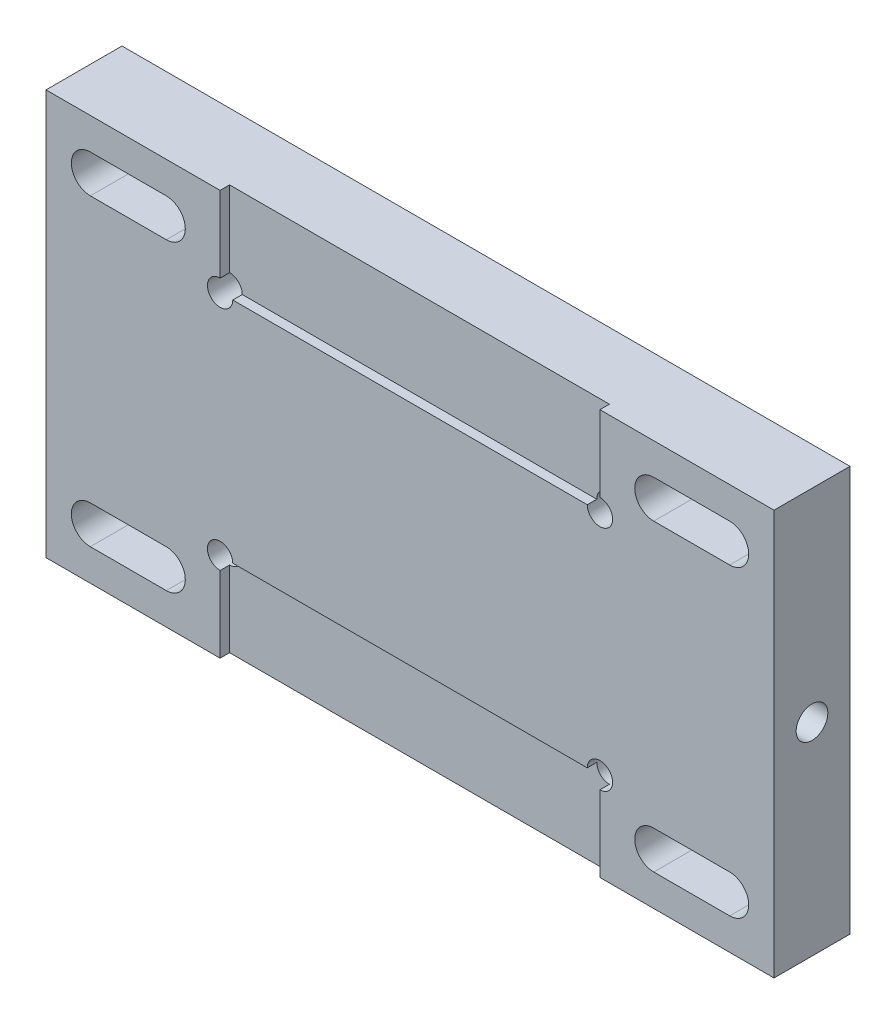
SolidWorks part; units mm, degrees
ref_plane "前视基准面" through (0, 0, 0) normal (0, 0, 1) x (1, 0, 0)
ref_plane "上视基准面" through (0, 0, 0) normal (0, 1, 0) x (1, 0, 0)
ref_plane "右视基准面" through (0, 0, 0) normal (1, 0, 0) x (0, 0, -1)
sketch "草图1" plane through (0, 0, 0) normal (0, 0, 1) x (1, 0, 0)
  line L1 (-57.5, -32) -> (57.5, -32)
  line L2 (-57.5, -32) -> (-57.5, 32)
  line L3 (-57.5, 32) -> (57.5, 32)
  line L4 (57.5, -32) -> (57.5, 32)
  line L5 (-57.5, -32) -> (57.5, 32) construction
  line L6 (-57.5, 32) -> (57.5, -32) construction
  point P0 (0, 0)
  dimension "D1" = 64
  dimension "D2" = 115
extrude "凸台-拉伸1" add sketch "草图1" along normal mid plane 12
sketch "草图2" plane through (0, 0, 6) normal (0, 0, 1) x (1, 0, 0)
  line L0 (57.5, 32) -> (-57.5, 32) construction
  line L1 (-30, 18) -> (30, 18)
  line L2 (-30, 18) -> (-30, 32)
  line L3 (-30, 32) -> (30, 32)
  line L4 (30, 18) -> (30, 32)
  line L5 (-30, 18) -> (30, 32) construction
  line L6 (-30, 32) -> (30, 18) construction
  point P0 (0, 25)
  dimension "D1" = 60
  dimension "D2" = 14
extrude "切除-拉伸1" cut sketch "草图2" against normal blind 1.5
sketch "草图3" plane through (0, 0, 6) normal (0, 0, 1) x (1, 0, 0)
  circle A0 centre (-30, 18) radius 2
  circle A1 centre (30, 18) radius 2
  dimension "D1" = 4
extrude "切除-拉伸2" cut sketch "草图3" against normal through all both and the other way through all
mirror "镜向1" about plane through (0, 0, 0) normal (0, 1, 0) of "切除-拉伸2", "切除-拉伸1"
sketch "草图4" plane through (0, 0, 6) normal (0, 0, 1) x (1, 0, 0)
  line L0 (-50.5, 24) -> (-38.5, 24) construction
  line L1 (-50.5, 27) -> (-38.5, 27)
  line L2 (-50.5, 21) -> (-38.5, 21)
  line L3 (-30, 32) -> (-57.5, 32) construction
  line L4 (-57.5, 32) -> (-57.5, -32) construction
  line L5 (0, 0) -> (0, 32) construction
  line L6 (30, 32) -> (-30, 32) construction
  line L7 (0, 0) -> (-57.5, 0) construction
  line L8 (50.5, 24) -> (38.5, 24) construction
  line L9 (50.5, 27) -> (38.5, 27)
  line L10 (50.5, 21) -> (38.5, 21)
  line L11 (-50.5, -24) -> (-38.5, -24) construction
  line L12 (-50.5, -27) -> (-38.5, -27)
  line L13 (-50.5, -21) -> (-38.5, -21)
  line L14 (50.5, -24) -> (38.5, -24) construction
  line L15 (50.5, -27) -> (38.5, -27)
  line L16 (50.5, -21) -> (38.5, -21)
  arc A0 (-50.5, 27) -> (-50.5, 21) centre (-50.5, 24) ccw
  arc A1 (-38.5, 21) -> (-38.5, 27) centre (-38.5, 24) ccw
  arc A2 (50.5, 27) -> (50.5, 21) centre (50.5, 24) cw
  arc A3 (38.5, 21) -> (38.5, 27) centre (38.5, 24) cw
  arc A4 (-50.5, -27) -> (-50.5, -21) centre (-50.5, -24) cw
  arc A5 (-38.5, -21) -> (-38.5, -27) centre (-38.5, -24) cw
  arc A6 (50.5, -27) -> (50.5, -21) centre (50.5, -24) ccw
  arc A7 (38.5, -21) -> (38.5, -27) centre (38.5, -24) ccw
  point P2 (-44.5, 24)
  point P19 (44.5, 24)
  point P26 (-44.5, -24)
  point P33 (44.5, -24)
  dimension "D1" = 3
  dimension "D2" = 12
  dimension "D3" = 5
  dimension "D4" = 7
extrude "切除-拉伸3" cut sketch "草图4" against normal up to next
hole_wizard "M6 螺纹孔1" positions "3D草图1" profile "草图5" tap size "M6" standard "GB"
sketch3d "3D草图1"
  line L0 (57.5, 0, 6) -> (57.5, 0, -6)
  line L1 (57.5, -32, 6) -> (57.5, 32, 6) construction
  line L2 (57.5, -32, -6) -> (57.5, 32, -6) construction
  point P0 (57.5, 0, 0)
sketch "草图5" plane through (57.5, 0, 0) normal (0, 1, 0) x (0, 0, -1)
  line L0 (0, 0) -> (0, 19.5022)
  line L1 (0, 19.5022) -> (2.5, 18)
  line L2 (2.5, 18) -> (2.5, 0)
  line L5 (2.5, 0) -> (0, 0)
  line L10 (0, 19.5022) -> (-2.5, 18) construction
  line L11 (0, -6.35) -> (0, 107.95) construction
  dimension "螺纹孔钻头直径" = 5
  dimension "螺纹孔钻头深度" = 18
  dimension "导头角度" = 118
cosmetic thread "孔螺蚊线1" parameters "D1"=15, "D2"=6
